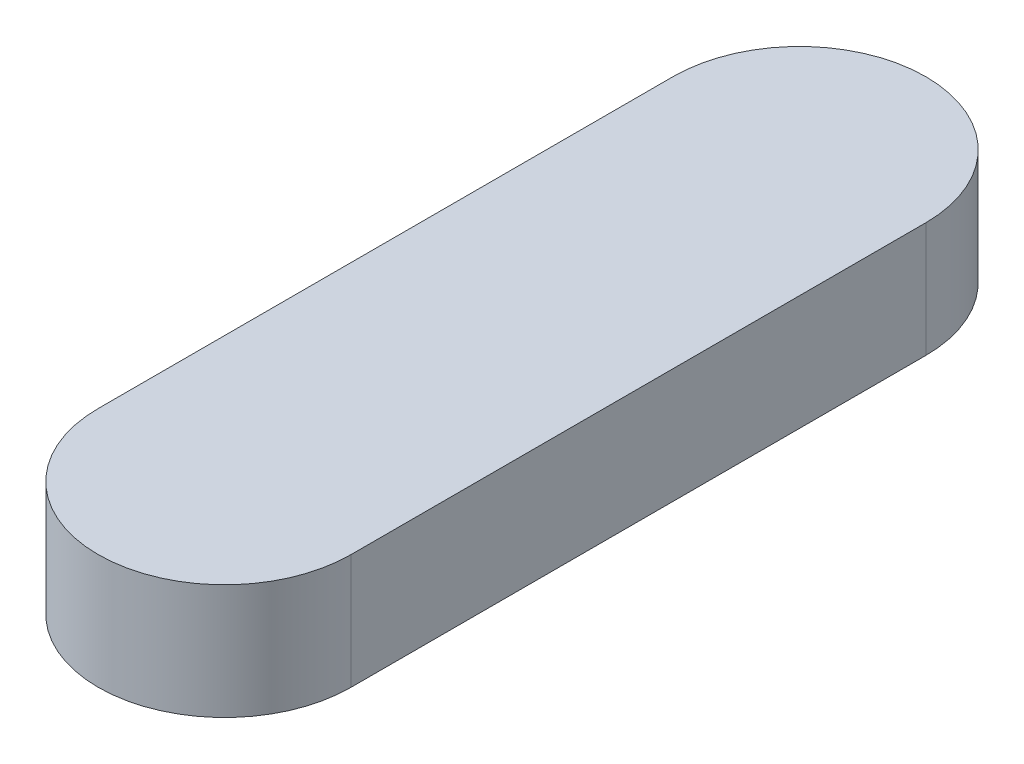
SolidWorks part; units mm, degrees
ref_plane "Front Plane" through (0, 0, 0) normal (0, 0, 1) x (1, 0, 0)
ref_plane "Top Plane" through (0, 0, 0) normal (0, 1, 0) x (1, 0, 0)
ref_plane "Right Plane" through (0, 0, 0) normal (1, 0, 0) x (0, 0, -1)
sketch "Sketch1" plane through (0, 0, 0) normal (0, 1, 0) x (1, 0, 0)
  line L0 (0, -25) -> (0, 25) construction
  line L1 (-11, -25) -> (-11, 25)
  line L2 (11, -25) -> (11, 25)
  arc A0 (-11, -25) -> (11, -25) centre (0, -25) ccw
  arc A1 (11, 25) -> (-11, 25) centre (0, 25) ccw
  point P2 (0, 0)
  dimension "D1" = 22
  dimension "D2" = 50
extrude "Boss-Extrude1" add sketch "Sketch1" along normal blind 10
